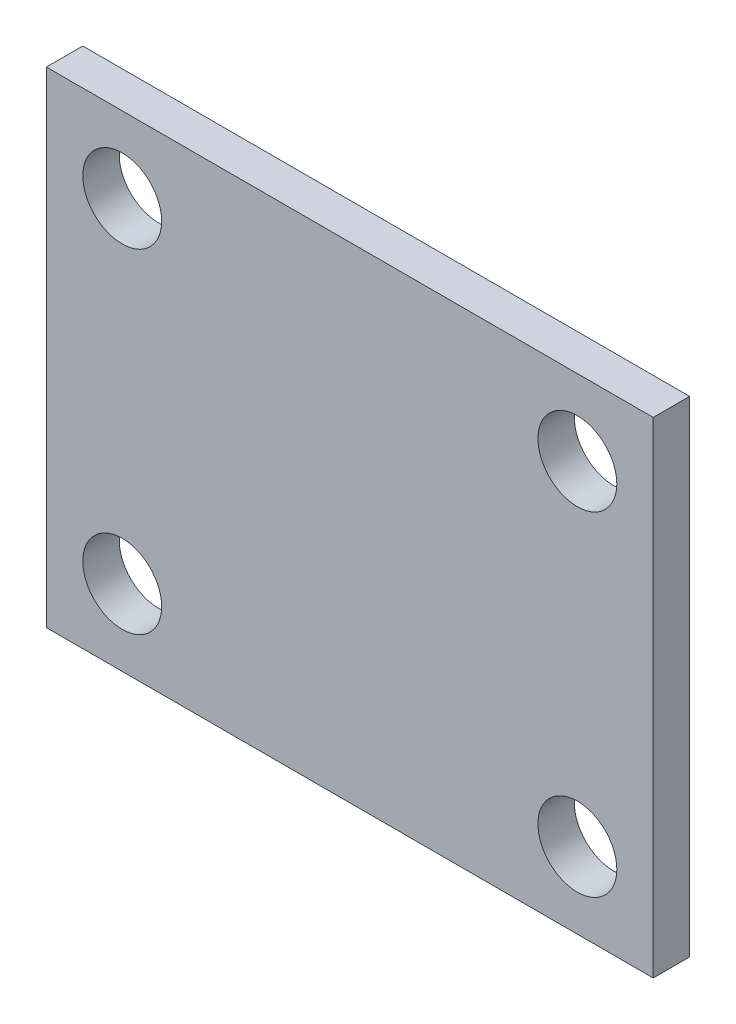
from build123d import *

# Parameters (mm, degrees)
SKETCH1_W           = 100
SKETCH1_H           = 80
BOSS_EXTRUDE1_DEPTH = 6
SKETCH2_R           = 6.5
CUT_EXTRUDE1_DEPTH  = 6


with BuildPart() as part:
    # Sketch1 → Boss-Extrude1 (new body)
    with BuildSketch(Plane.XY):
        Rectangle(SKETCH1_W, SKETCH1_H)
    extrude(amount=BOSS_EXTRUDE1_DEPTH)

    # Sketch2 → Cut-Extrude1 (cut)
    with BuildSketch(Plane.XY.offset(6)):
        with Locations((-37.5, 27.5)):
            Circle(SKETCH2_R)
        with Locations((37.5, 27.5)):
            Circle(SKETCH2_R)
        with Locations((37.5, -27.5)):
            Circle(SKETCH2_R)
        with Locations((-37.5, -27.5)):
            Circle(SKETCH2_R)
    extrude(amount=-CUT_EXTRUDE1_DEPTH, mode=Mode.SUBTRACT)


solid = part.part
